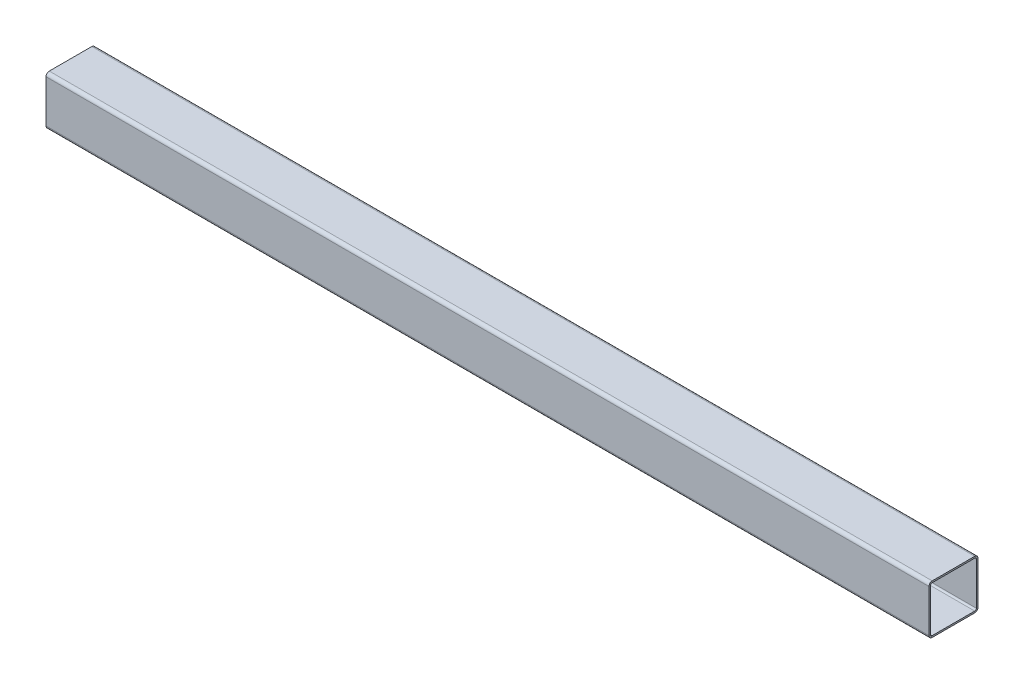
from build123d import *

# Parameters (mm, degrees)
GB_6728_1986_150_X_150_X_5_1_DEPTH = 2700


with BuildPart() as part:
    # Sketch1 → Gb／6728-1986方形空心型钢 150 X 150 X 5(1) (new body)
    with BuildSketch(Plane.YZ.offset(-1350)):
        with BuildLine():
            Line((-65, -75), (65, -75))
            ThreePointArc((65, -75), (72.071067812, -72.071067812), (75, -65))
            Line((75, -65), (75, 65))
            ThreePointArc((75, 65), (72.071067812, 72.071067812), (65, 75))
            Line((65, 75), (-65, 75))
            ThreePointArc((-65, 75), (-72.071067812, 72.071067812), (-75, 65))
            Line((-75, 65), (-75, -65))
            ThreePointArc((-75, -65), (-72.071067812, -72.071067812), (-65, -75))
        make_face()
        with BuildLine():
            Line((-65, -70), (65, -70))
            ThreePointArc((65, -70), (68.535533906, -68.535533906), (70, -65))
            Line((70, -65), (70, 65))
            ThreePointArc((70, 65), (68.535533906, 68.535533906), (65, 70))
            Line((65, 70), (-65, 70))
            ThreePointArc((-65, 70), (-68.535533906, 68.535533906), (-70, 65))
            Line((-70, 65), (-70, -65))
            ThreePointArc((-70, -65), (-68.535533906, -68.535533906), (-65, -70))
        make_face(mode=Mode.SUBTRACT)
    extrude(amount=GB_6728_1986_150_X_150_X_5_1_DEPTH)


solid = part.part
